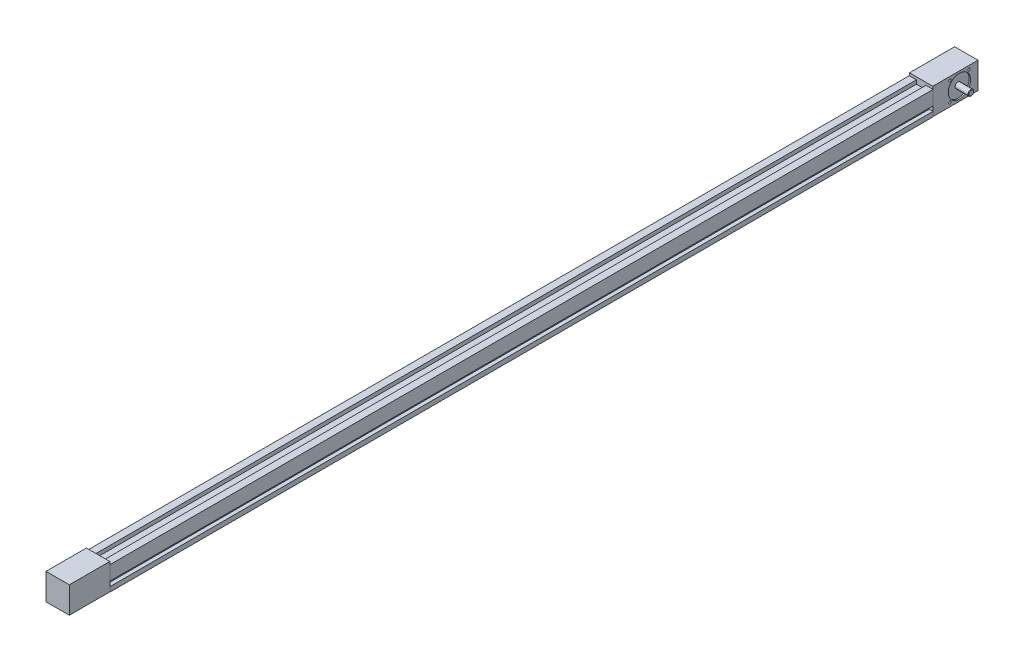
from build123d import *

# Parameters (mm, degrees)
EXTRUDE_670_DEPTH        = 1730
SKETCH_2_W               = 49
SKETCH_2_H               = 55.5
EXTRUDE_1_DEPTH          = 85
SKETCH_4_W               = 49
SKETCH_4_H               = 55.5
EXTRUDE_3_DEPTH          = 95
SKETCH_9_R               = 23.5
CUT_EXTRUDE_5_DEPTH      = 3
SKETCH_10_R              = 6
EXTRUDE_4_DEPTH          = 28
CHAMFER_1_SIZE           = 1
PATTERN_CIRCULAR_1_COUNT = 4


with BuildPart() as part:
    # 草图1 → Extrude 670 (new body)
    with BuildSketch(Plane.XY):
        Polygon((15, 50), (15, 42), (35, 42), (35, 50), (50, 50), (50, 20), (42, 20), (42, 10), (50, 10), (50, 0), (0, 0), (0, 10), (8, 10), (8, 20), (0, 20), (0, 50), align=None)
    extrude(amount=EXTRUDE_670_DEPTH)

    # 草图2 → 凸台-拉伸1 (add)
    with BuildSketch(Plane.XY.offset(1730)):
        with Locations((25, 27.75)):
            Rectangle(SKETCH_2_W, SKETCH_2_H)
    extrude(amount=EXTRUDE_1_DEPTH)

    # 草图4 → 凸台-拉伸3 (add)
    with BuildSketch(Plane(origin=(0, 0, 0), x_dir=(-1, 0, 0), z_dir=(0, 0, -1))):
        with Locations((-25, 27.75)):
            Rectangle(SKETCH_4_W, SKETCH_4_H)
    extrude(amount=EXTRUDE_3_DEPTH)

    # 草图9 → 切除-拉伸5 (cut)
    with BuildSketch(Plane(origin=(49.5, 0, 0), x_dir=(0, 0, -1), z_dir=(1, 0, 0))):
        with Locations((56, 27.75)):
            Circle(SKETCH_9_R)
    extrude(amount=-CUT_EXTRUDE_5_DEPTH, mode=Mode.SUBTRACT)

    # 草图10 → 凸台-拉伸4 (add)
    with BuildSketch(Plane(origin=(46.5, 0, 0), x_dir=(0, 0, -1), z_dir=(1, 0, 0))):
        with Locations((56, 27.75)):
            Circle(SKETCH_10_R)
    extrude(amount=EXTRUDE_4_DEPTH)

    # 倒角1
    chamfer_1_edges = [part.edges().sort_by_distance(p)[0] for p in [
        (74.5, 27.75, -50),
    ]]
    chamfer(chamfer_1_edges, length=CHAMFER_1_SIZE)

    # 草图12 → M5 螺纹孔1 (revolve, cut)
    with BuildSketch(Plane(origin=(50, 47.75, -76), x_dir=(0, 0, -1), z_dir=(0, 1, 0))):
        Polygon((0, 0), (0, 15.2618073), (2.1, 14), (2.1, 10), (2.5, 10), (2.5, 0), align=None)
    hole_wizard_m5_1 = revolve(axis=Axis((56.35, 47.75, -76), (-1, 0, 0)), mode=Mode.SUBTRACT)

    # 阵列(圆周)1: M5 螺纹孔1 ×4 about axis
    pattern_circular_1_axis = Axis((0, 27.75, -56), (1, 0, 0))
    for i in range(1, PATTERN_CIRCULAR_1_COUNT):
        add(hole_wizard_m5_1.rotate(pattern_circular_1_axis, i * 360 / PATTERN_CIRCULAR_1_COUNT), mode=Mode.SUBTRACT)


solid = part.part
